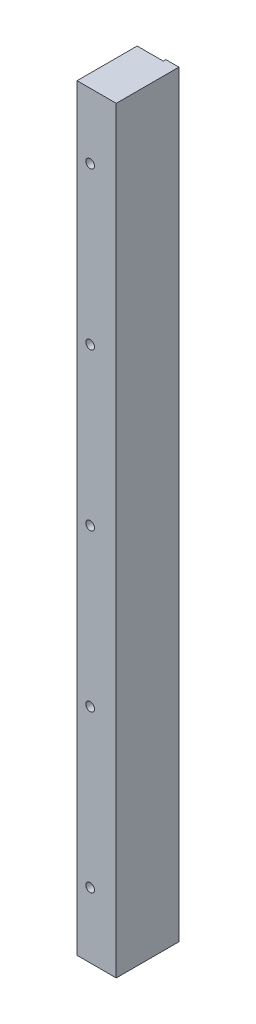
SolidWorks part; units mm, degrees
ref_plane "前视基准面" through (0, 0, 0) normal (0, 0, 1) x (1, 0, 0)
ref_plane "上视基准面" through (0, 0, 0) normal (0, 1, 0) x (1, 0, 0)
ref_plane "右视基准面" through (0, 0, 0) normal (1, 0, 0) x (0, 0, -1)
sketch "草图1" plane through (0, 0, 0) normal (0, 0, 1) x (1, 0, 0)
  line L1 (15, -290) -> (-15, -290)
  line L2 (15, -290) -> (15, 290)
  line L3 (15, 290) -> (-15, 290)
  line L4 (-15, -290) -> (-15, 290)
  line L5 (15, -290) -> (-15, 290) construction
  line L6 (15, 290) -> (-15, -290) construction
  point P0 (0, 0)
  dimension "D1" = 30
  dimension "D2" = 580
extrude "凸台-拉伸1" add sketch "草图1" along normal blind 48
sketch "草图2" plane through (0, 0, 0) normal (0, 0, -1) x (-1, 0, 0)
  line L0 (15, -290) -> (-15, -290) construction
  line L1 (-5, 290) -> (15, 290)
  line L2 (-5, 290) -> (-5, -290)
  line L3 (-5, -290) -> (15, -290)
  line L4 (15, 290) -> (15, -290)
  dimension "D1" = 20
extrude "切除-拉伸1" cut sketch "草图2" against normal blind 2
hole_wizard "M5 螺纹孔1" positions "草图3" profile "草图4" tap size "M5" standard "GB"
sketch "草图3" plane through (0, 0, 2) normal (0, 0, -1) x (-1, 0, 0)
  point P0 (5, 270)
sketch "草图4" plane through (-5, 270, 2) normal (1, 0, 0) x (0, 1, 0)
  line L0 (0, 0) -> (0, 13.6618)
  line L1 (0, 13.6618) -> (2.1, 12.4)
  line L2 (2.1, 12.4) -> (2.1, 0)
  line L5 (2.1, 0) -> (0, 0)
  line L10 (0, 13.6618) -> (-2.1, 12.4) construction
  line L11 (0, -6.35) -> (0, 107.95) construction
  dimension "螺纹孔钻头直径" = 4.2
  dimension "螺纹孔钻头深度" = 12.4
  dimension "导头角度" = 118
pattern_linear "阵列(线性)1" count 10 spacing 60 along (0, -1, 0) of "M5 螺纹孔1"
hole_wizard "打孔尺寸(%根据)内六角圆柱头螺钉的类型1" positions "草图5" profile "草图6" counterbore size "M6" standard "GB" end condition up to next
sketch "草图5" plane through (0, 0, 2) normal (0, 0, -1) x (-1, 0, 0)
  line L0 (5, 270) -> (5, 210) construction
  point P8 (5, 240)
sketch "草图6" plane through (-5, 240, 2) normal (1, 0, 0) x (0, 1, 0)
  line L0 (0, 0) -> (0, 46)
  line L1 (0, 46) -> (3.3, 46)
  line L3 (3.3, 46) -> (3.3, 6.8)
  line L4 (3.3, 6.8) -> (5.5, 6.8)
  line L5 (5.5, 6.8) -> (5.5, 0)
  line L7 (5.5, 0) -> (0, 0)
  line L11 (0, -6.35) -> (0, 107.95) construction
  dimension "通孔孔直径" = 6.6
  dimension "通孔孔深度" = 46
  dimension "柱形沉头孔直径" = 11
  dimension "柱形沉头孔深度" = 6.8
pattern_linear "阵列(线性)2" count 5 spacing 120 along (0, -1, 0) of "打孔尺寸(%根据)内六角圆柱头螺钉的类型1"
